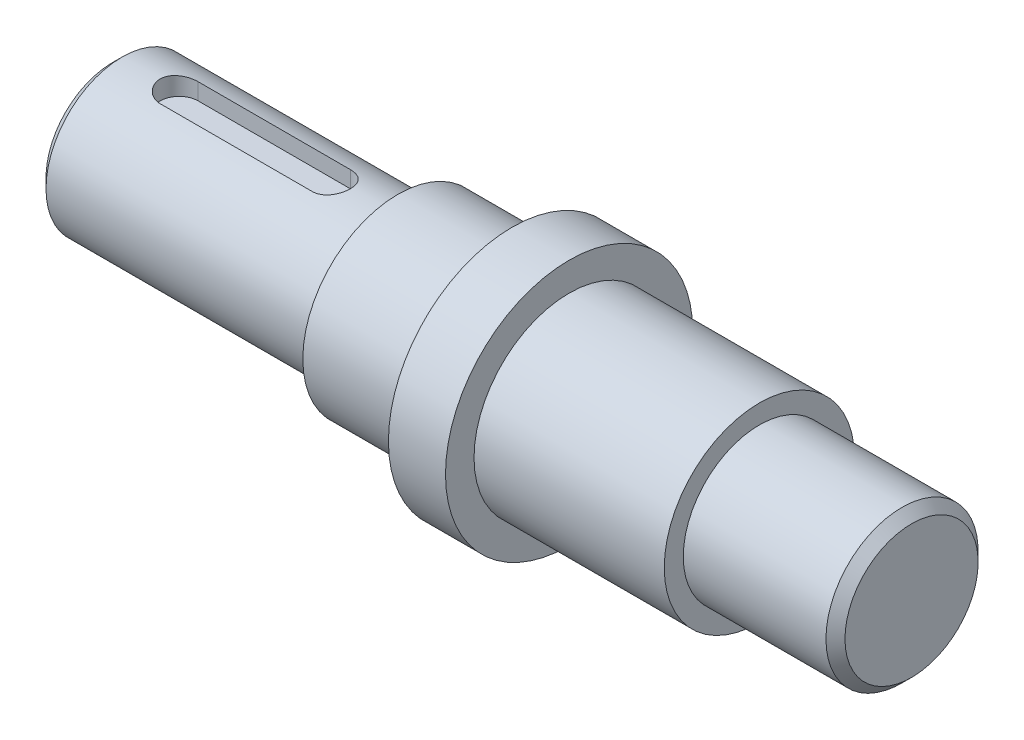
from build123d import *

# Parameters (mm, degrees)
CUT_EXTRUDE_3_DEPTH = 1
SKETCH_5_R          = 1.5
CUT_EXTRUDE_4_DEPTH = 10
CHAMFER_1_SIZE      = 0.5
CHAMFER_2_SIZE      = 0.5


with BuildPart() as part:
    # 草图1 → 旋转2 (revolve)
    with BuildSketch(Plane.XY, mode=Mode.PRIVATE) as revolve_2_sk:
        Polygon((-23.267570956, 0), (-23.267570956, 4), (-8.267570956, 4), (-8.267570956, 5), (-2.267570956, 5), (-2.267570956, 6.5), (0.732429044, 6.5), (0.732429044, 5), (10.732429044, 5), (10.732429044, 4), (18.732429044, 4), (18.732429044, 0), align=None)
    revolve(revolve_2_sk.sketch.rotate(Axis((-82.03072058, 0, 0), (1, 0, 0)), 90), axis=Axis((-82.03072058, 0, 0), (1, 0, 0)))

    # 草图4 → 切除-拉伸3 (cut)
    with BuildSketch(Plane(origin=(0, 4, 0), x_dir=(1, 0, 0), z_dir=(0, 1, 0))):
        with BuildLine():
            Line((-19.767570956, 1), (-11.767570956, 1))
            ThreePointArc((-11.767570956, 1), (-10.767570956, 0), (-11.767570956, -1))
            Line((-11.767570956, -1), (-19.767570956, -1))
            ThreePointArc((-19.767570956, -1), (-20.767570956, 0), (-19.767570956, 1))
        make_face()
    extrude(amount=-CUT_EXTRUDE_3_DEPTH, mode=Mode.SUBTRACT)

    # 草图5 → 切除-拉伸4 (cut)
    with BuildSketch(Plane.ZY.offset(23.267570956)):
        Circle(SKETCH_5_R)
    extrude(amount=-CUT_EXTRUDE_4_DEPTH, mode=Mode.SUBTRACT)

    # 倒角1
    chamfer_1_edges = [part.edges().sort_by_distance(p)[0] for p in [
        (-23.267570956, 0, -4),
    ]]
    chamfer(chamfer_1_edges, length=CHAMFER_1_SIZE)

    # 倒角2
    chamfer_2_edges = [part.edges().sort_by_distance(p)[0] for p in [
        (18.732429044, 0, -4),
    ]]
    chamfer(chamfer_2_edges, length=CHAMFER_2_SIZE)


solid = part.part
